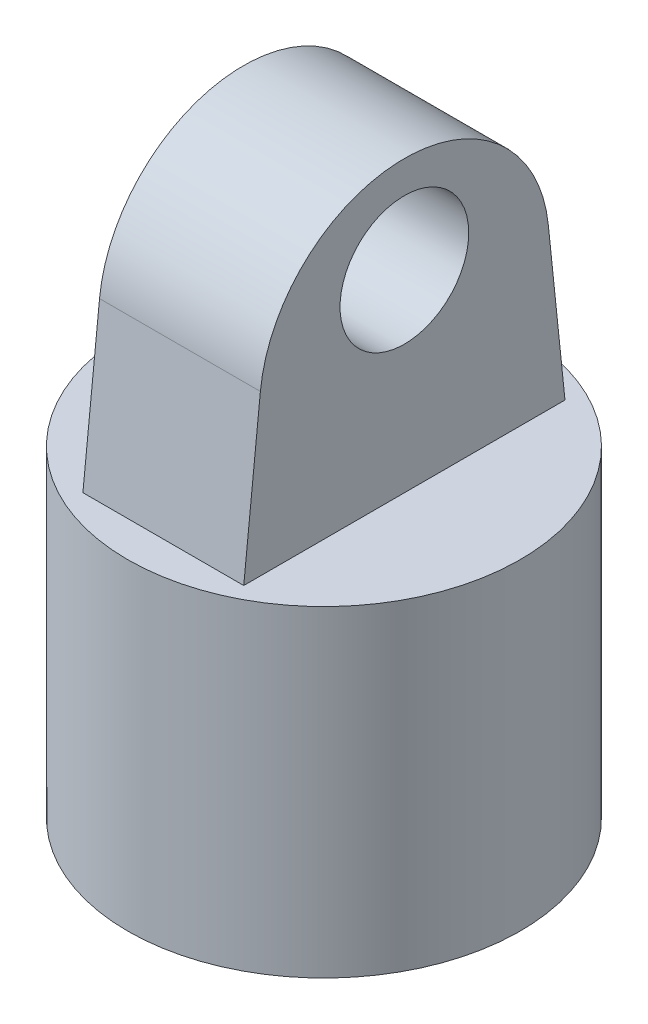
from build123d import *

# Parameters (mm, degrees)
SKETCH1_R           = 6.1
BOSS_EXTRUDE1_DEPTH = 10
BOSS_EXTRUDE2_DEPTH = 2.5
SKETCH3_R           = 2
CUT_EXTRUDE1_DEPTH  = 22.729473072
SKETCH4_R           = 5.6
CUT_EXTRUDE2_DEPTH  = 5
CHAMFER1_SIZE       = 0.72


with BuildPart() as part:
    # Sketch1 → Boss-Extrude1 (new body)
    with BuildSketch(Plane(origin=(0, 0, 0), x_dir=(1, 0, 0), z_dir=(0, 1, 0))):
        with Locations(Location((0, 0, 0), (0, 0, 270))):
            Circle(SKETCH1_R)
    extrude(amount=BOSS_EXTRUDE1_DEPTH)

    # Sketch2 → Boss-Extrude2 (add, symmetric)
    with BuildSketch(Plane(origin=(0, 0, 0), x_dir=(0, 0, -1), z_dir=(1, 0, 0))):
        with BuildLine():
            Line((-4.992659986, 10), (-4.475823522, 14.965836668))
            ThreePointArc((-4.475823522, 14.965836668), (0, 19), (4.475823522, 14.965836668))
            Line((4.475823522, 14.965836668), (4.992659986, 10))
            Line((4.992659986, 10), (-4.992659986, 10))
        make_face()
    extrude(amount=BOSS_EXTRUDE2_DEPTH, both=True)

    # Sketch3 → Cut-Extrude1 (cut, through all)
    with BuildSketch(Plane(origin=(2.5, 0, 0), x_dir=(0, 0, -1), z_dir=(1, 0, 0))):
        with Locations((0, 16)):
            Circle(SKETCH3_R)
    extrude(amount=-CUT_EXTRUDE1_DEPTH, mode=Mode.SUBTRACT)

    # Sketch4 → Cut-Extrude2 (cut)
    with BuildSketch(Plane.XZ):
        with Locations(Location((0, 0, 0), (0, 0, 270))):
            Circle(SKETCH4_R)
    extrude(amount=-CUT_EXTRUDE2_DEPTH, mode=Mode.SUBTRACT)

    # Chamfer1
    chamfer1_edges = [part.edges().sort_by_distance(p)[0] for p in [
        (0, 5, 5.6),
    ]]
    chamfer(chamfer1_edges, length=CHAMFER1_SIZE)


solid = part.part
